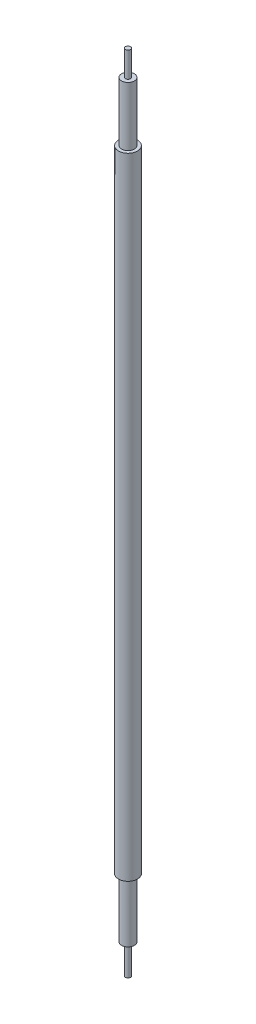
from build123d import *

# Parameters (mm, degrees)
SKETCH1_R           = 1.125
BOSS_EXTRUDE1_DEPTH = 74.7
SKETCH2_R           = 0.75
BOSS_EXTRUDE2_DEPTH = 7
SKETCH3_R           = 0.3
BOSS_EXTRUDE3_DEPTH = 3.5
BOSS_EXTRUDE4_START = 7
SKETCH4_R           = 0.75
BOSS_EXTRUDE4_DEPTH = 7
SKETCH5_R           = 0.299867591
BOSS_EXTRUDE5_DEPTH = 3


with BuildPart() as part:
    # Sketch1 → Boss-Extrude1 (new body)
    with BuildSketch(Plane(origin=(0, 0, 0), x_dir=(1, 0, 0), z_dir=(0, 1, 0))):
        with Locations(Location((0, 0, 0), (0, 0, 270))):
            Circle(SKETCH1_R)
    extrude(amount=BOSS_EXTRUDE1_DEPTH)

    # Sketch2 → Boss-Extrude2 (add)
    with BuildSketch(Plane.XZ):
        with Locations(Location((0, 0, 0), (0, 0, 90))):
            Circle(SKETCH2_R)
    extrude(amount=BOSS_EXTRUDE2_DEPTH)

    # Sketch3 → Boss-Extrude3 (add)
    with BuildSketch(Plane.XZ.offset(7)):
        with Locations(Location((0, 0, 0), (0, 0, 270))):
            Circle(SKETCH3_R)
    extrude(amount=BOSS_EXTRUDE3_DEPTH)

    # Sketch4 → Boss-Extrude4 (add)
    with BuildSketch(Plane(origin=(0, 74.7, 0), x_dir=(1, 0, 0), z_dir=(0, 1, 0)).offset(BOSS_EXTRUDE4_START)):
        with Locations(Location((0, 0, 0), (0, 0, 270))):
            Circle(SKETCH4_R)
    extrude(amount=-BOSS_EXTRUDE4_DEPTH)

    # Sketch5 → Boss-Extrude5 (add)
    with BuildSketch(Plane(origin=(0, 81.7, 0), x_dir=(1, 0, 0), z_dir=(0, 1, 0))):
        with Locations(Location((0, 0, 0), (0, 0, 270))):
            Circle(SKETCH5_R)
    extrude(amount=BOSS_EXTRUDE5_DEPTH)


solid = part.part
